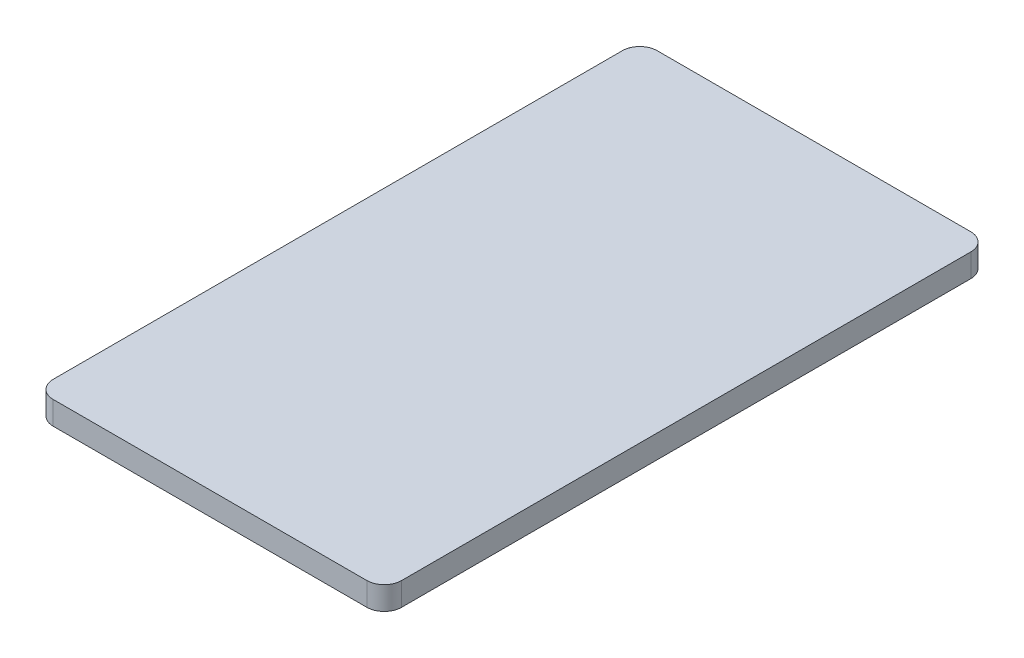
SolidWorks part; units mm, degrees
ref_plane "Front Plane" through (0, 0, 0) normal (0, 0, 1) x (1, 0, 0)
ref_plane "Top Plane" through (0, 0, 0) normal (0, 1, 0) x (1, 0, 0)
ref_plane "Right Plane" through (0, 0, 0) normal (1, 0, 0) x (0, 0, -1)
sketch "Sketch 1" plane through (0, 0, 0) normal (0, 1, 0) x (1, 0, 0)
  line L0 (0, 129.8246) -> (0, -147.3684) construction
  line L1 (-161.4035, 0) -> (194.7368, 0) construction
  line L2 (135, 260) -> (-135, 260)
  line L3 (-150, 245) -> (-150, -245)
  line L4 (135, -260) -> (-135, -260)
  line L5 (150, 245) -> (150, -245)
  circle A0 centre (-90, 200) radius 15 construction
  arc A1 (-135, 260) -> (-150, 245) centre (-135, 245) ccw
  arc A2 (-135, -260) -> (-150, -245) centre (-135, -245) cw
  arc A3 (135, -260) -> (150, -245) centre (135, -245) ccw
  arc A4 (135, 260) -> (150, 245) centre (135, 245) cw
  point P7 (150, 0)
  point P9 (0, 260)
  point P15 (-150, 0)
  point P22 (0, -260)
  dimension "D3" = 30
  dimension "D4" = 15
  dimension "D5" = 60
  dimension "D6" = 60
  dimension "D1" = 300
  dimension "D2" = 520
extrude "Boss-Extrude 1" add sketch "Sketch 1" along normal blind 20
